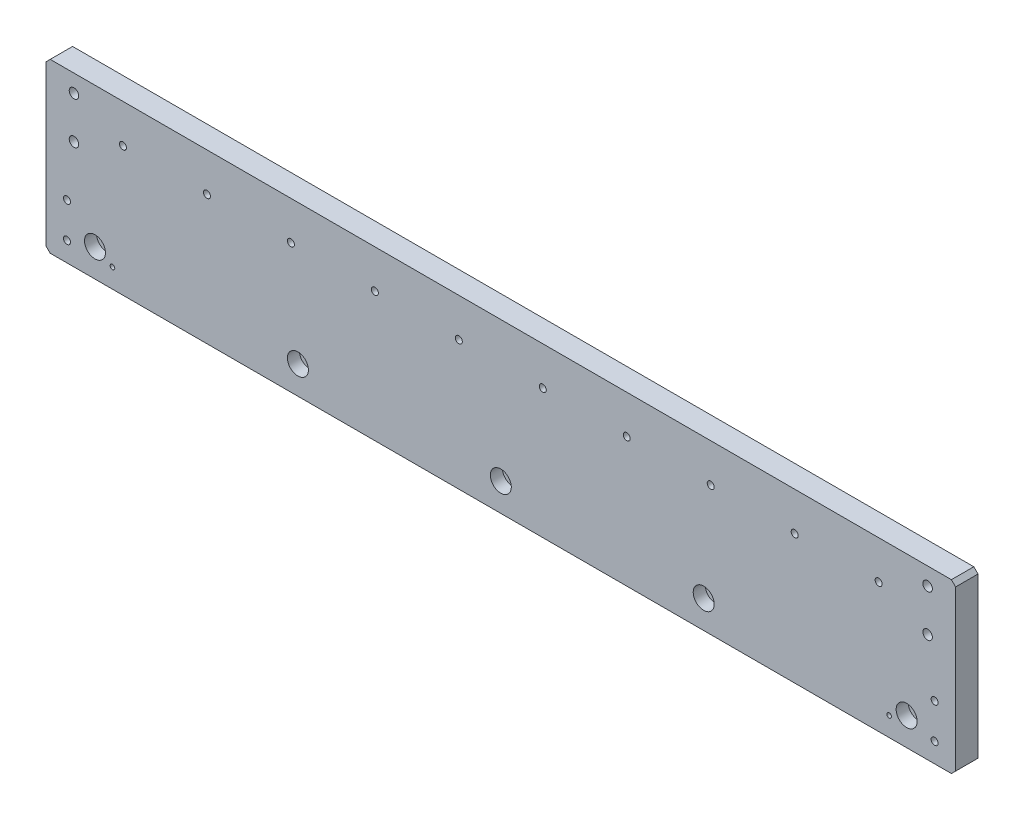
SolidWorks part; units mm, degrees
ref_plane "前视基准面" through (0, 0, 0) normal (0, 0, 1) x (1, 0, 0)
ref_plane "上视基准面" through (0, 0, 0) normal (0, 1, 0) x (1, 0, 0)
ref_plane "右视基准面" through (0, 0, 0) normal (1, 0, 0) x (0, 0, -1)
sketch "草图1" plane through (0, 0, 0) normal (0, 0, 1) x (1, 0, 0)
  line L1 (-335, 70) -> (335, 70)
  line L2 (-335, 70) -> (-335, -70)
  line L3 (-335, -70) -> (335, -70)
  line L4 (335, 70) -> (335, -70)
  line L5 (-335, 70) -> (335, -70) construction
  line L6 (-335, -70) -> (335, 70) construction
  point P0 (0, 0)
  dimension "D1" = 670
  dimension "D2" = 140
extrude "凸台-拉伸1" add sketch "草图1" along normal blind 16
hole_wizard "M8 螺纹孔1" positions "草图4" profile "草图2" tap size "M8" standard "ISO" end condition through all
sketch "草图4" plane through (0, 0, 16) normal (0, 0, 1) x (1, 0, 0)
  line L0 (335, 70) -> (-335, 70) construction
  line L1 (-335, 70) -> (-335, -70) construction
  line L2 (0, 83.7605) -> (0, -85.3934) construction
  point P0 (-305, 57.5)
  point P2 (-305, 27.5)
  point P15 (305, 27.5)
  point P16 (305, 57.5)
  dimension "D1" = 12.5
  dimension "D2" = 30
  dimension "D3" = 30
sketch "草图2" plane through (-305, 57.5, 16) normal (1, 0, 0) x (0, -1, 0)
  line L0 (0, 0) -> (0, 16)
  line L1 (0, 16) -> (3.4, 16)
  line L2 (3.4, 16) -> (3.4, 0)
  line L5 (3.4, 0) -> (0, 0)
  line L11 (0, -6.35) -> (0, 107.95) construction
  dimension "通孔螺纹孔钻头直径" = 6.8
  dimension "通孔螺纹孔钻头深度" = 16
cosmetic thread "孔螺蚊线1" parameters "D2"=8
cosmetic thread "孔螺蚊线2" parameters "D2"=8
cosmetic thread "孔螺蚊线3" parameters "D2"=8
cosmetic thread "孔螺蚊线4" parameters "D2"=8
hole_wizard "M6 螺纹孔1" positions "草图9" profile "草图8" tap size "M6" standard "ISO" end condition through all
sketch "草图9" plane through (0, 0, 16) normal (0, 0, 1) x (1, 0, 0)
  line L0 (335, 70) -> (-335, 70) construction
  line L1 (-335, 70) -> (-335, -70) construction
  point P0 (-270, 42.5)
  point P16 (-210, 42.5)
  point P17 (-150, 42.5)
  point P18 (-90, 42.5)
  point P19 (-30, 42.5)
  point P20 (30, 42.5)
  point P21 (90, 42.5)
  point P22 (150, 42.5)
  point P23 (210, 42.5)
  point P24 (270, 42.5)
  dimension "D1" = 27.5
  dimension "65" = 65
  dimension "D3" = 10
sketch "草图8" plane through (-270, 42.5, 16) normal (1, 0, 0) x (0, -1, 0)
  line L0 (0, 0) -> (0, 16)
  line L1 (0, 16) -> (2.5, 16)
  line L2 (2.5, 16) -> (2.5, 0)
  line L5 (2.5, 0) -> (0, 0)
  line L11 (0, -6.35) -> (0, 107.95) construction
  dimension "通孔螺纹孔钻头直径" = 5
  dimension "通孔螺纹孔钻头深度" = 16
cosmetic thread "孔螺蚊线5" parameters "D2"=6
cosmetic thread "孔螺蚊线6" parameters "D2"=6
cosmetic thread "孔螺蚊线7" parameters "D2"=6
cosmetic thread "孔螺蚊线8" parameters "D2"=6
cosmetic thread "孔螺蚊线9" parameters "D2"=6
cosmetic thread "孔螺蚊线10" parameters "D2"=6
cosmetic thread "孔螺蚊线11" parameters "D2"=6
cosmetic thread "孔螺蚊线12" parameters "D2"=6
cosmetic thread "孔螺蚊线13" parameters "D2"=6
cosmetic thread "孔螺蚊线14" parameters "D2"=6
hole_wizard "M8 六角凹头螺钉的柱形沉头孔1" positions "草图15" profile "草图14" counterbore size "M8" standard "ISO" end condition through all
sketch "草图15" plane through (0, 0, 16) normal (0, 0, 1) x (1, 0, 0)
  line L0 (335, -70) -> (335, 70) construction
  line L1 (-335, -70) -> (335, -70) construction
  point P0 (290, -30)
  point P13 (145, -30)
  point P14 (0, -30)
  point P15 (-145, -30)
  point P16 (-290, -30)
  point P17 (-435, -30)
  dimension "D1" = 45
  dimension "D2" = 40
  dimension "D3" = 6
sketch "草图14" plane through (290, -30, 16) normal (1, 0, 0) x (0, -1, 0)
  line L0 (0, 0) -> (0, 16)
  line L1 (0, 16) -> (4.5, 16)
  line L3 (4.5, 16) -> (4.5, 8.6)
  line L4 (4.5, 8.6) -> (7.5, 8.6)
  line L5 (7.5, 8.6) -> (7.5, 0)
  line L7 (7.5, 0) -> (0, 0)
  line L11 (0, -6.35) -> (0, 107.95) construction
  dimension "通孔孔直径" = 9
  dimension "通孔孔深度" = 16
  dimension "柱形沉头孔直径" = 15
  dimension "柱形沉头孔深度" = 8.6
sketch "草图16" plane through (0, 0, 16) normal (0, 0, 1) x (1, 0, 0)
  line L1 (-335, -50) -> (335, -50)
  line L2 (-335, -50) -> (-335, -70)
  line L3 (-335, -70) -> (335, -70)
  line L4 (335, -50) -> (335, -70)
  line L5 (335, -70) -> (335, 70) construction
  line L6 (-335, -70) -> (335, -70) construction
  line L7 (-335, 70) -> (-335, -70) construction
  dimension "D1" = 20
extrude "切除-拉伸1" cut sketch "草图16" against normal through all
sketch "草图19" plane through (0, 0, 16) normal (0, 0, 1) x (1, 0, 0)
  line L1 (-335, 70) -> (-325, 70)
  line L2 (-335, 70) -> (-335, -50)
  line L3 (-335, -50) -> (-325, -50)
  line L4 (-325, 70) -> (-325, -50)
  line L5 (335, -50) -> (-335, -50) construction
  dimension "D1" = 10
extrude "切除-拉伸2" cut sketch "草图19" against normal through all
mirror "镜向1" about plane through (0, 0, 0) normal (1, 0, 0) of "切除-拉伸2"
chamfer "倒角1" distance 3 angle 45 4 edges at (325, 70, 8) (-325, 70, 8) (325, -50, 8) (-325, -50, 8)
hole_wizard "M6 螺纹孔2" positions "草图25" profile "草图24" tap size "M6" standard "ISO" end condition through all
sketch "草图25" plane through (0, 0, 16) normal (0, 0, 1) x (1, 0, 0)
  point P0 (-310, -11)
  point P3 (-310, -36)
  point P18 (310, -11)
  point P21 (310, -36)
sketch "草图24" plane through (-310, -11, 16) normal (1, 0, 0) x (0, -1, 0)
  line L0 (0, 0) -> (0, 16)
  line L1 (0, 16) -> (2.5, 16)
  line L2 (2.5, 16) -> (2.5, 0)
  line L5 (2.5, 0) -> (0, 0)
  line L11 (0, -6.35) -> (0, 107.95) construction
  dimension "通孔螺纹孔钻头直径" = 5
  dimension "通孔螺纹孔钻头深度" = 16
cosmetic thread "孔螺蚊线18" parameters "D2"=6
cosmetic thread "孔螺蚊线24" parameters "D2"=6
cosmetic thread "孔螺蚊线27" parameters "D2"=6
cosmetic thread "孔螺蚊线29" parameters "D2"=6
hole_wizard "M4 螺纹孔1" positions "草图27" profile "草图26" tap size "M4" standard "ISO" end condition up to next
sketch "草图27" plane through (0, 0, 16) normal (0, 0, 1) x (1, 0, 0)
  point P0 (277.5, -36.25)
  point P3 (-277.5, -36.25)
sketch "草图26" plane through (277.5, -36.25, 16) normal (1, 0, 0) x (0, -1, 0)
  line L0 (0, 0) -> (0, 16)
  line L1 (0, 16) -> (1.65, 16)
  line L2 (1.65, 16) -> (1.65, 0)
  line L5 (1.65, 0) -> (0, 0)
  line L11 (0, -6.35) -> (0, 107.95) construction
  dimension "通孔螺纹孔钻头直径" = 3.3
  dimension "通孔螺纹孔钻头深度" = 16
cosmetic thread "孔螺蚊线30" parameters "D2"=4
cosmetic thread "孔螺蚊线31" parameters "D2"=4
